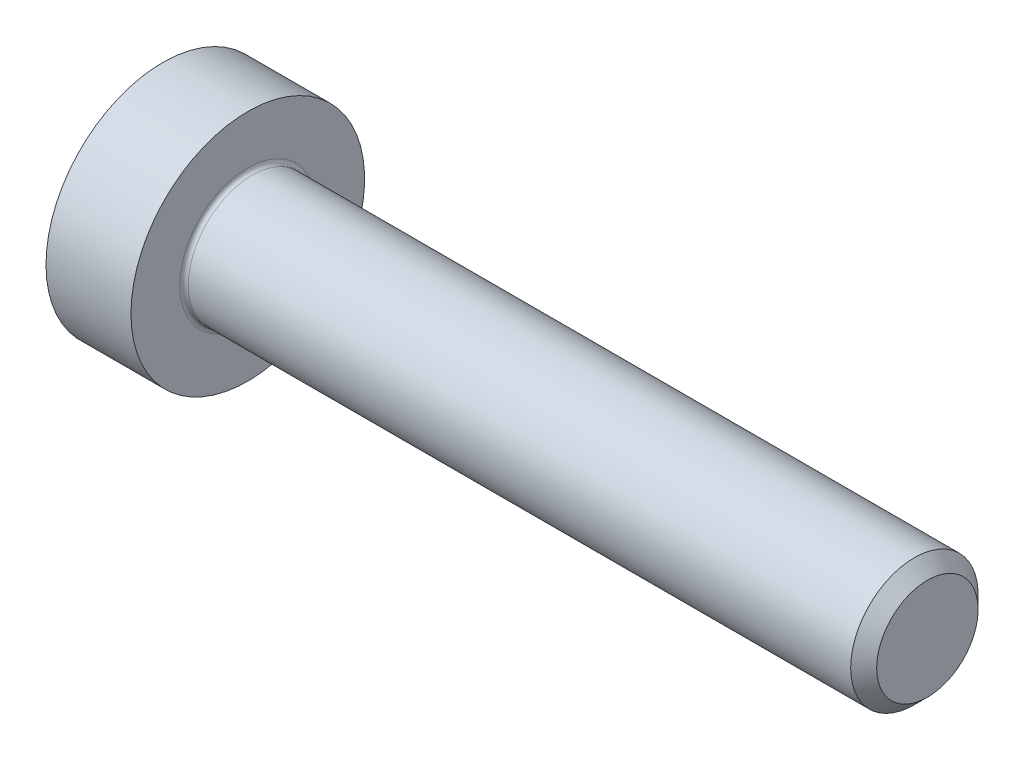
from build123d import *

# Parameters (mm, degrees)
CUT_EXTRUDE1_DEPTH = 1.5


with BuildPart() as part:
    # Sketch1 → Revolve1 (revolve)
    with BuildSketch(Plane.XY, mode=Mode.PRIVATE) as revolve1_sk:
        with BuildLine():
            Line((-2, 0), (-2, 2.75))
            Line((-2, 2.75), (0, 2.75))
            Line((0, 2.75), (0, 1.6))
            ThreePointArc((0, 1.6), (0.029289322, 1.529289322), (0.1, 1.5))
            Line((0.1, 1.5), (15.6935, 1.5))
            Line((15.6935, 1.5), (16, 1.1935))
            Line((16, 1.1935), (16, 0))
            Line((16, 0), (-2, 0))
        make_face()
    revolve(revolve1_sk.sketch.rotate(Axis((16, 0, 0), (-1, 0, 0)), 270), axis=Axis((16, 0, 0), (-1, 0, 0)))

    # Sketch2 → Cut-Revolve1 (revolve, cut)
    with BuildSketch(Plane.XY, mode=Mode.PRIVATE) as cut_revolve1_sk:
        Polygon((-2, 0), (-2, 1), (-0.5, 1), (-0.136029766, 0), align=None)
    revolve(cut_revolve1_sk.sketch.rotate(Axis((0, 0, 0), (-1, 0, 0)), 270), axis=Axis((0, 0, 0), (-1, 0, 0)), mode=Mode.SUBTRACT)

    # Sketch3 → Cut-Extrude1 (cut)
    with BuildSketch(Plane(origin=(-2, 0, 0), x_dir=(0, 0, -1), z_dir=(1, 0, 0))):
        Polygon((-1, 0.577350269), (-1, -0.577350269), (0, -1.154700538), (1, -0.577350269), (1, 0.577350269), (0, 1.154700538), align=None)
    extrude(amount=CUT_EXTRUDE1_DEPTH, mode=Mode.SUBTRACT)


solid = part.part
